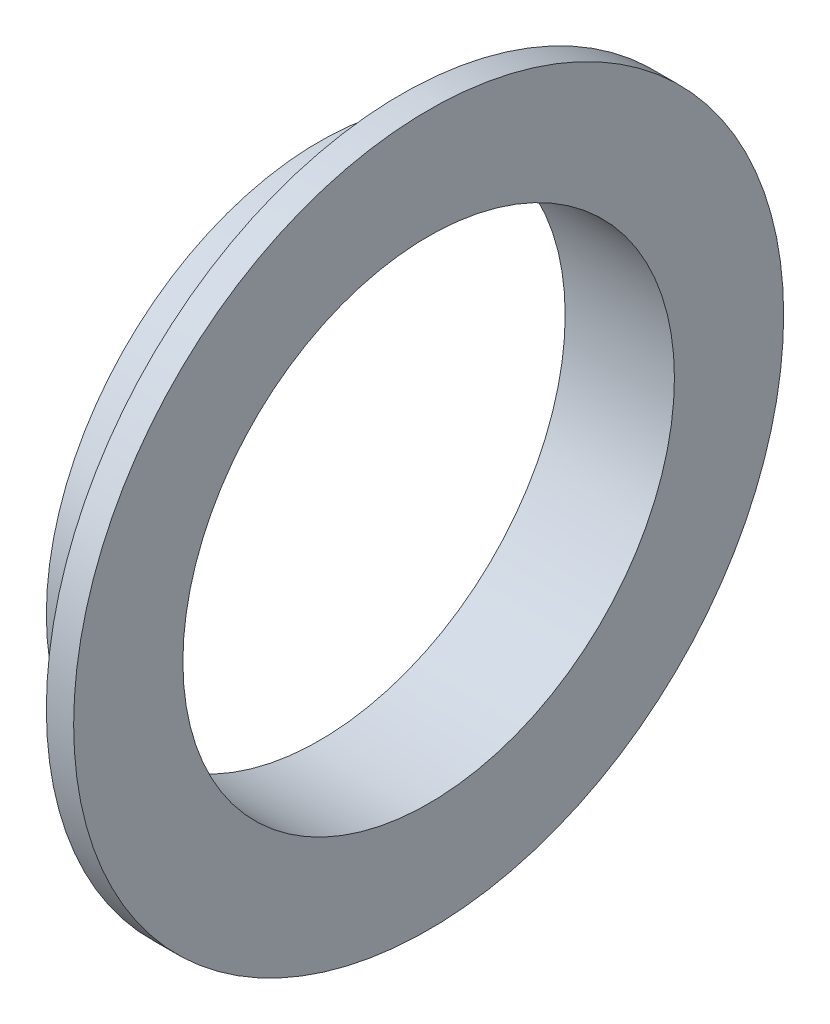
from build123d import *


with BuildPart() as part:
    # 草图1 → 旋转1 (revolve)
    with BuildSketch(Plane(origin=(0, 0, 0), x_dir=(1, 0, 0), z_dir=(0, 1, 0)), mode=Mode.PRIVATE) as revolve_1_sk:
        Polygon((0, 9), (0, 10), (3, 10), (3, 13), (4, 13), (4, 9), align=None)
    revolve(revolve_1_sk.sketch.rotate(Axis((-397.809040607, 0, 0), (1, 0, 0)), 180), axis=Axis((-397.809040607, 0, 0), (1, 0, 0)))


solid = part.part
